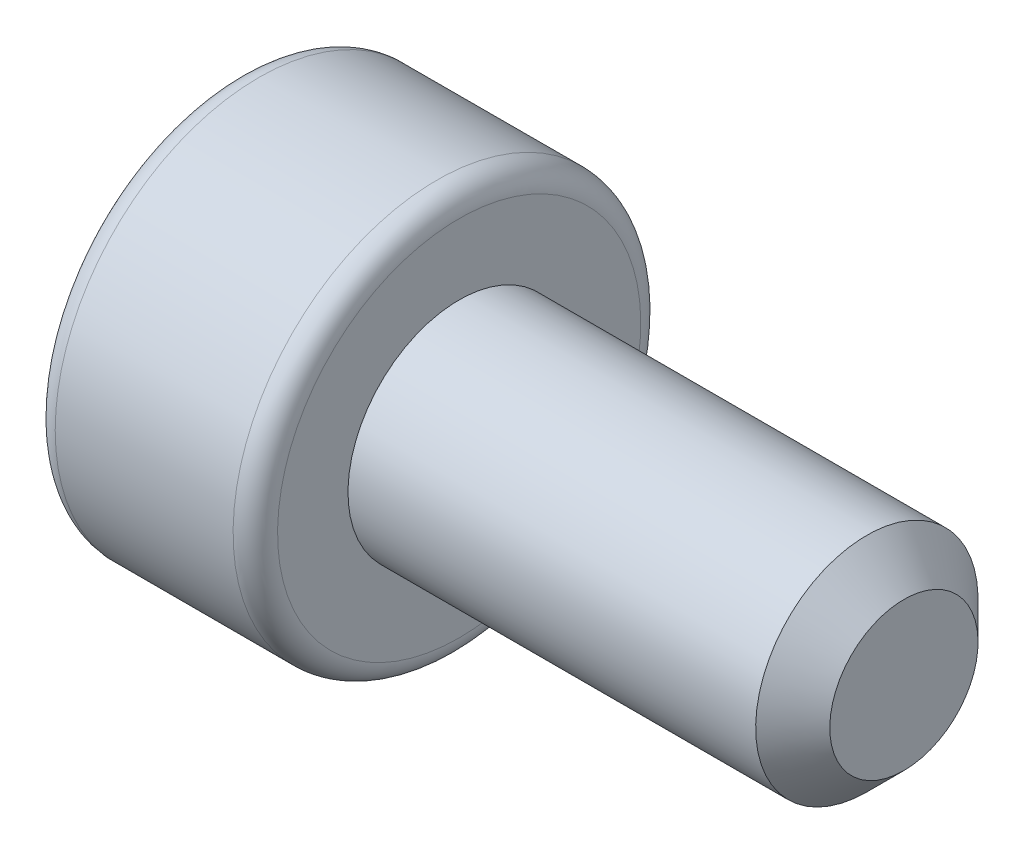
SolidWorks part; units mm, degrees
material "AISI 304"
ref_plane "Front Plane" through (0, 0, 0) normal (0, 0, 1) x (1, 0, 0)
ref_plane "Top Plane" through (0, 0, 0) normal (0, 1, 0) x (1, 0, 0)
ref_plane "Right Plane" through (0, 0, 0) normal (1, 0, 0) x (0, 0, -1)
sketch "Sketch1" plane through (0, 0, 0) normal (0, 0, 1) x (1, 0, 0)
  line L0 (-4.7092, 0) -> (9, 0) construction
  line L1 (0, 0) -> (0, 2.75)
  line L2 (0, 2.75) -> (3, 2.75)
  line L3 (3, 2.75) -> (3, 1.5)
  line L4 (3, 1.5) -> (9, 1.5)
  line L5 (9, 1.5) -> (9, 0)
  line L6 (9, 0) -> (0, 0)
  dimension "D1" = 5.5
  dimension "D2" = 3
  dimension "D3" = 3
  dimension "D4" = 6
revolve "Revolve1" add sketch "Sketch1" angle 360 about L0
cosmetic thread "Cosmetic Thread1" parameters "D2"=3
sketch "Sketch4" plane through (0, 0, 0) normal (-1, 0, 0) x (0, 0, 1)
  line L1 (-1.4434, 0) -> (-0.7217, -1.25)
  line L2 (-0.7217, -1.25) -> (0.7217, -1.25)
  line L3 (0.7217, -1.25) -> (1.4434, 0)
  line L4 (1.4434, 0) -> (0.7217, 1.25)
  line L5 (0.7217, 1.25) -> (-0.7217, 1.25)
  line L6 (-0.7217, 1.25) -> (-1.4434, 0)
  circle A0 centre (0, 0) radius 1.25 construction
  dimension "D1" = 2.5
extrude "Cut-Extrude1" cut sketch "Sketch4" against normal blind 1.3
fillet "Fillet1" radius 0.3 2 edges at (3, -2.75, 0) (0, -2.75, 0)
chamfer "Chamfer1" distance 0.1 angle 80 6 edges at (0, -0.625, -1.0825) (0, -1.25, 0) (0, -0.625, 1.0825) (0, 0.625, 1.0825) (0, 1.25, 0) (0, 0.625, -1.0825)
chamfer "Chamfer2" distance 0.5 angle 45 1 edges at (9, -1.5, 0)
